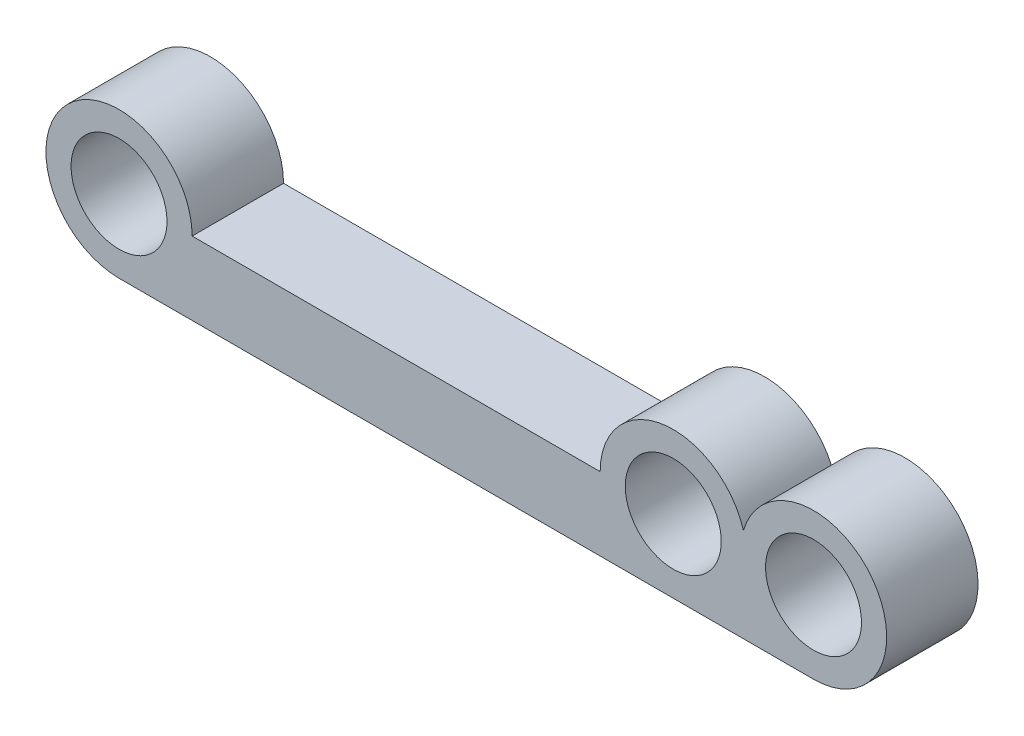
from build123d import *
from build123d.topology import SkipClean

# Parameters (mm, degrees)
BOSS_EXTRUDE1_DEPTH          = 5
SKETCH2_R                    = 2.5
BOSS_EXTRUDE2_DEPTH          = 7
SKETCH4_R                    = 2.5
BOSS_EXTRUDE4_DEPTH          = 9
SKETCH10_R                   = 2.5
BOSS_EXTRUDE6_DEPTH          = 5
SKETCH13_W                   = 0.75
SKETCH13_H                   = 0.75
CUT_REVOLVE1_ANGLE           = 45
CUT_REVOLVE1_OTHER_WAY_ANGLE = 45
SKETCH15_W                   = 0.75
SKETCH15_H                   = 0.75
CUT_REVOLVE2_ANGLE           = 45
CUT_REVOLVE2_OTHER_WAY_ANGLE = 45
SKETCH17_R                   = 4
BOSS_EXTRUDE7_DEPTH          = 5
SKETCH18_R                   = 2.930859256
CUT_EXTRUDE1_DEPTH           = 7
SKETCH19_R                   = 2.625
CUT_EXTRUDE2_DEPTH           = 7
SKETCH20_R                   = 4
BOSS_EXTRUDE8_DEPTH          = 5
SKETCH21_R                   = 2.625
CUT_EXTRUDE3_DEPTH           = 50.162013496
SKETCH23_R                   = 4
BOSS_EXTRUDE9_DEPTH          = 5
SKETCH24_R                   = 2.625
CUT_EXTRUDE4_DEPTH           = 15
CUT_EXTRUDE5_DEPTH           = 10
CUT_EXTRUDE6_DEPTH           = 48.390965078
BOSS_EXTRUDE10_DEPTH         = 5


with BuildPart() as part:
    # Sketch1 → Boss-Extrude1 (new body)
    with BuildSketch(Plane.XY):
        with BuildLine():
            Line((1, 0), (44, 0))
            ThreePointArc((44, 0), (44.707106781, -0.292893219), (45, -1))
            Line((45, -1), (45, -4))
            ThreePointArc((45, -4), (44.707106781, -4.707106781), (44, -5))
            Line((44, -5), (1, -5))
            ThreePointArc((1, -5), (0.292893219, -4.707106781), (0, -4))
            Line((0, -4), (0, -1))
            ThreePointArc((0, -1), (0.292893219, -0.292893219), (1, 0))
        make_face()
    extrude(amount=BOSS_EXTRUDE1_DEPTH)

    # Sketch2 → Boss-Extrude2 (add)
    with BuildSketch(Plane(origin=(0, 0, 0), x_dir=(-1, 0, 0), z_dir=(0, 0, -1))):
        with Locations(Location((-42.676049222, -2.5, 0), (0, 0, 158.369487395))):
            Circle(SKETCH2_R)
    extrude(amount=BOSS_EXTRUDE2_DEPTH)

    # Sketch4 → Boss-Extrude4 (add)
    with BuildSketch(Plane.XY.offset(5)):
        with Locations(Location((35, -2.5, 0), (0, 0, 270))):
            Circle(SKETCH4_R)
    extrude(amount=BOSS_EXTRUDE4_DEPTH)

    # Sketch10 → Boss-Extrude6 (add)
    with BuildSketch(Plane.XY.offset(5)):
        with Locations(Location((4.676049222, -2.5, 0), (0, 0, 270))):
            Circle(SKETCH10_R)
    extrude(amount=BOSS_EXTRUDE6_DEPTH)

    # Sketch13 → Cut-Revolve1 (revolve, cut)
    with BuildSketch(Plane(origin=(35, 0, 1.995810748), x_dir=(0, 1, 0), z_dir=(1, 0, 0))):
        with Locations((-0.375, 8.375)):
            Rectangle(SKETCH13_W, SKETCH13_H)
        with Locations((-4.625, 8.375)):
            Rectangle(SKETCH13_W, SKETCH13_H)
    revolve(axis=Axis((35, -2.5, 15.995810748), (0, 0, -1)), revolution_arc=CUT_REVOLVE1_ANGLE, mode=Mode.SUBTRACT)

    # Sketch13 → Cut-Revolve1 other way (revolve, cut)
    with BuildSketch(Plane(origin=(35, 0, 1.995810748), x_dir=(0, 1, 0), z_dir=(1, 0, 0))):
        with Locations((-0.375, 8.375)):
            Rectangle(SKETCH13_W, SKETCH13_H)
        with Locations((-4.625, 8.375)):
            Rectangle(SKETCH13_W, SKETCH13_H)
    revolve(axis=Axis((35, -2.5, 15.995810748), (0, 0, 1)), revolution_arc=CUT_REVOLVE1_OTHER_WAY_ANGLE, mode=Mode.SUBTRACT)

    # Sketch15 → Cut-Revolve2 (revolve, cut)
    with BuildSketch(Plane(origin=(42.676049222, 0, -1.99986967), x_dir=(0, 1, 0), z_dir=(-1, 0, 0))):
        with Locations((-0.375, 3.375)):
            Rectangle(SKETCH15_W, SKETCH15_H)
        with Locations((-4.625, 3.375)):
            Rectangle(SKETCH15_W, SKETCH15_H)
    revolve(axis=Axis((42.676049222, -2.5, -8.99986967), (0, 0, 1)), revolution_arc=CUT_REVOLVE2_ANGLE, mode=Mode.SUBTRACT)

    # Sketch15 → Cut-Revolve2 other way (revolve, cut)
    with BuildSketch(Plane(origin=(42.676049222, 0, -1.99986967), x_dir=(0, 1, 0), z_dir=(-1, 0, 0))):
        with Locations((-0.375, 3.375)):
            Rectangle(SKETCH15_W, SKETCH15_H)
        with Locations((-4.625, 3.375)):
            Rectangle(SKETCH15_W, SKETCH15_H)
    revolve(axis=Axis((42.676049222, -2.5, -8.99986967), (0, 0, -1)), revolution_arc=CUT_REVOLVE2_OTHER_WAY_ANGLE, mode=Mode.SUBTRACT)

    # Sketch17 → Boss-Extrude7 (add)
    with BuildSketch(Plane.XY.offset(5)):
        with Locations((42.676049222, -2.5)):
            Circle(SKETCH17_R)
    extrude(amount=-BOSS_EXTRUDE7_DEPTH)

    # Sketch18 → Cut-Extrude1 (cut)
    with BuildSketch(Plane(origin=(0, 0, -7), x_dir=(-1, 0, 0), z_dir=(0, 0, -1))):
        with Locations((-42.676049222, -2.5)):
            Circle(SKETCH18_R)
    extrude(amount=-CUT_EXTRUDE1_DEPTH, mode=Mode.SUBTRACT)

    # Sketch19 → Cut-Extrude2 (cut)
    with BuildSketch(Plane.XY.offset(5)):
        with Locations((42.676049222, -2.5)):
            Circle(SKETCH19_R)
    extrude(amount=-CUT_EXTRUDE2_DEPTH, mode=Mode.SUBTRACT)

    # Sketch20 → Boss-Extrude8 (add)
    with BuildSketch(Plane(origin=(0, 0, 0), x_dir=(-1, 0, 0), z_dir=(0, 0, -1))):
        with Locations((-35, -2.5)):
            Circle(SKETCH20_R)
    extrude(amount=-BOSS_EXTRUDE8_DEPTH)

    # Sketch21 → Cut-Extrude3 (cut, through all)
    with BuildSketch(Plane(origin=(0, 0, 0), x_dir=(-1, 0, 0), z_dir=(0, 0, -1))):
        with Locations((-35, -2.5)):
            Circle(SKETCH21_R)
    extrude(amount=-CUT_EXTRUDE3_DEPTH, mode=Mode.SUBTRACT)

    # Sketch23 → Boss-Extrude9 (add)
    with BuildSketch(Plane.XY.offset(5)):
        with Locations((4.676049222, -2.5)):
            Circle(SKETCH23_R)
    extrude(amount=-BOSS_EXTRUDE9_DEPTH)

    # Sketch24 → Cut-Extrude4 (cut)
    with BuildSketch(Plane.XY.offset(10)):
        with Locations((4.676049222, -2.5)):
            Circle(SKETCH24_R)
    extrude(amount=-CUT_EXTRUDE4_DEPTH, mode=Mode.SUBTRACT)

    # Sketch25 → Cut-Extrude5 (cut)
    with BuildSketch(Plane.XY.offset(5)):
        with BuildLine():
            Line((1.553550223, -5), (-1.854692679, -7.728778219))
            Line((-1.854692679, -7.728778219), (-3.436521983, -2.874938814))
            Line((-3.436521983, -2.874938814), (-1.53654244, 1.593813071))
            Line((-1.53654244, 1.593813071), (0.676049222, 3.037797523))
            Line((0.676049222, 3.037797523), (1.553550223, 0))
            ThreePointArc((1.553550223, 0), (0.676049222, -2.5), (1.553550223, -5))
        make_face()
    extrude(amount=-CUT_EXTRUDE5_DEPTH, mode=Mode.SUBTRACT)

    # Sketch26 → Cut-Extrude6 (cut, through all)
    with SkipClean():  # the faces are left unmerged after this step: merging them gives an invalid solid
        with BuildSketch(Plane.XY.offset(5)):
            Polygon((31, 2.88382286), (31, 2.910088177), (31.877501001, 0), (7.798548222, 0), align=None)
            with BuildLine():
                Line((39.403739803, 2.542373737), (38.122498999, 0))
                Line((38.122498999, 0), (39.553550223, 0))
                ThreePointArc((39.553550223, 0), (39.704808809, 0.178008664), (39.866200483, 0.346884273))
                Line((39.866200483, 0.346884273), (39.403739803, 2.542373737))
            make_face()
            with BuildLine():
                ThreePointArc((31.877501001, 0), (31.225745372, -1.175235115), (31, -2.5))
                Line((31, -2.5), (8.676049222, -2.5))
                ThreePointArc((8.676049222, -2.5), (8.450303851, -1.175235115), (7.798548222, 0))
                Line((7.798548222, 0), (31.877501001, 0))
            make_face()
            with BuildLine():
                Line((39.553550223, 0), (38.122498999, 0))
                ThreePointArc((38.122498999, 0), (38.547347694, -0.651669851), (38.838024611, -1.373249325))
                ThreePointArc((38.838024611, -1.373249325), (39.128701529, -0.651669851), (39.553550223, 0))
            make_face()
        extrude(amount=-CUT_EXTRUDE6_DEPTH, mode=Mode.SUBTRACT)

    # Sketch27 → Boss-Extrude10 (add, through all)
    with SkipClean():  # the faces are left unmerged after this step: merging them gives an invalid solid
        with BuildSketch(Plane.XY.offset(5)):
            Polygon((4.676049222, -6.5), (35, -6.5), (42.676049222, -6.5), (39.429079082, -3.966331103), (35, -5.966502381), (31.287082695, -3.966331103), (8.288836977, -3.966331103), align=None)
        extrude(amount=-BOSS_EXTRUDE10_DEPTH)


solid = part.part
